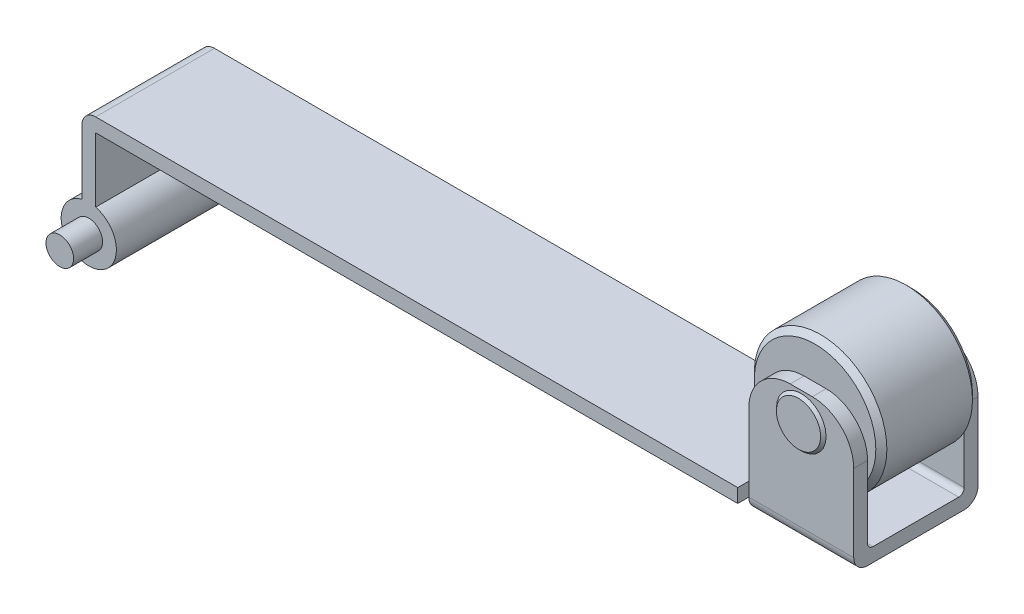
SolidWorks part; units mm, degrees
material "304"
ref_plane "前视基准面" through (0, 0, 0) normal (0, 0, 1) x (1, 0, 0)
ref_plane "上视基准面" through (0, 0, 0) normal (0, 1, 0) x (1, 0, 0)
ref_plane "右视基准面" through (0, 0, 0) normal (1, 0, 0) x (0, 0, -1)
sketch "草图1" plane through (0, 0, 0) normal (0, 0, 1) x (1, 0, 0)
  line L0 (0, 4.0987) -> (0, -2.2215) construction
  line L1 (-0.25, 3.3) -> (-0.25, 0.9682)
  line L2 (0.25, 3.8) -> (27.8, 3.8)
  line L3 (0.25, 3.3) -> (0.25, 0.9682)
  line L4 (0.25, 3.3) -> (27.8, 3.3)
  line L5 (27.8, 3.8) -> (27.8, 3.3)
  arc A0 (-0.25, 0.9682) -> (0.25, 0.9682) centre (0, 0) ccw
  arc A1 (-0.25, 3.3) -> (0.25, 3.8) centre (0.25, 3.3) cw
  arc A2 (0.25, 3.3) -> (0.25, 3.3) centre (0.25, 3.3) cw
  circle A3 centre (0, 0) radius 0.5
  dimension "D1" = 2
  dimension "D5" = 0.5
  dimension "D2" = 1
  dimension "D3" = 27.8
  dimension "D4" = 3.8
  dimension "D6" = 0.5
extrude "凸台-拉伸1" add sketch "草图1" along normal mid plane 4.3
sketch "草图2" plane through (0, 0, 0) normal (0, 0, 1) x (1, 0, 0)
  circle A0 centre (0, 0) radius 0.5
  circle A1 centre (0, 0) radius 0.5 construction
extrude "凸台-拉伸2" add sketch "草图2" along normal mid plane 6.4
sketch "草图3" plane through (27.8, 0, 0) normal (1, 0, 0) x (0, 0, -1)
  line L0 (0, 4.7957) -> (0, -0.8912) construction
  line L1 (-2.15, 3.8) -> (-1.75, 3.8)
  line L2 (-2.25, 3.3) -> (-2.25, 8.1)
  line L3 (-2.25, 8.1) -> (-1.75, 8.1)
  line L4 (-1.75, 3.8) -> (-1.75, 8.1)
  line L5 (2.15, 3.3) -> (2.25, 3.3)
  line L6 (2.15, 3.8) -> (2.15, 3.3)
  line L7 (1.75, 3.8) -> (1.75, 8.1)
  line L8 (2.25, 8.1) -> (1.75, 8.1)
  line L9 (-2.15, 3.3) -> (2.15, 3.3) construction
  line L10 (-2.15, 3.8) -> (2.15, 3.8) construction
  line L11 (-2.15, 3.8) -> (-2.15, 3.3)
  line L12 (-2.15, 3.3) -> (-2.25, 3.3)
  line L13 (2.25, 3.3) -> (2.25, 8.1)
  line L14 (2.15, 3.8) -> (1.75, 3.8)
  dimension "D1" = 0.5
  dimension "D2" = 4.8
  dimension "D3" = 4.5
extrude "凸台-拉伸3" add sketch "草图3" against normal blind 3.8
fillet "圆角2" radius 0.2 2 edges at (25.9, 3.8, 1.75) (25.9, 3.8, -1.75)
sketch "草图4" plane through (0, 3.8, 0) normal (0, 1, 0) x (1, 0, 0)
  line L0 (8.6269, 0) -> (19.5044, 0) construction
  line L1 (23.5, -2.25) -> (23.5, -1.6)
  line L2 (24, 2.25) -> (23.5, 2.25)
  line L3 (24, 2.25) -> (24, 1.6)
  line L4 (24, 1.6) -> (23.5, 1.6)
  line L5 (23.5, 2.25) -> (23.5, 1.6)
  line L6 (24, -1.6) -> (23.5, -1.6)
  line L7 (24, -2.25) -> (24, -1.6)
  line L8 (24, -2.25) -> (23.5, -2.25)
  dimension "D1" = 0.5
  dimension "D2" = 3.2
extrude "切除-拉伸1" cut sketch "草图4" against normal through all
fillet "圆角3" radius 0.5 2 edges at (25.9, 3.3, 2.25) (25.9, 3.3, -2.25)
sketch "草图5" plane through (0, 0, 0) normal (0, 0, 1) x (1, 0, 0)
  line L0 (25.9, 8.1) -> (25.9, 1.3698) construction
  line L1 (24, 8.1) -> (27.8, 8.1) construction
  line L3 (23.5, 3.8) -> (0.25, 3.8) construction
  circle A0 centre (25.9, 7.1) radius 1
  dimension "D1" = 2
  dimension "D2" = 3.3
extrude "凸台-拉伸4" add sketch "草图5" along normal mid plane 4.7 separate body
chamfer "倒角1" distance 0.2 angle 45 2 edges at (26.9, 7.1, 2.35) (26.9, 7.1, -2.35)
sketch "草图6" plane through (0, 0, 0) normal (0, 0, 1) x (1, 0, 0)
  circle A0 centre (25.9, 7.1) radius 2.4
  dimension "D1" = 4.8
extrude "凸台-拉伸5" add sketch "草图6" along normal mid plane 3.5 separate body
chamfer "倒角2" distance 0.2 angle 45 2 edges at (28.3, 7.1, -1.75) (28.3, 7.1, 1.75)
fillet "圆角4" radius 1.5 4 edges at (27.8, 8.1, 2) (24, 8.1, 2) (27.8, 8.1, -2) (24, 8.1, -2)
